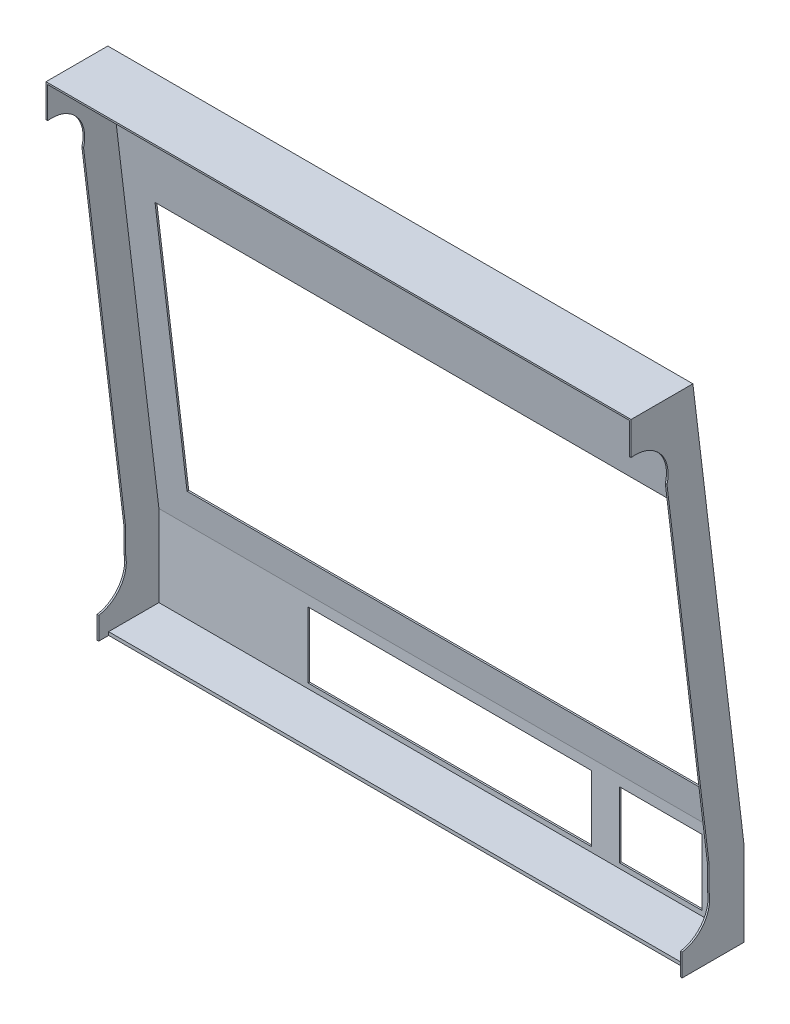
SolidWorks part; units mm, degrees
ref_plane "Front plane" through (0, 0, 0) normal (0, 0, 1) x (1, 0, 0)
ref_plane "Top plane" through (0, 0, 0) normal (0, 1, 0) x (1, 0, 0)
ref_plane "Right plane" through (0, 0, 0) normal (1, 0, 0) x (0, 0, -1)
sketch "Sketch1" plane through (0, 0, 0) normal (1, 0, 0) x (0, 0, -1)
  line L0 (0, 0) -> (-75, 0)
  line L1 (-75, 0) -> (-75, -40)
  line L2 (-13, -618) -> (-13, -590.821)
  line L3 (-31.4477, -90.1711) -> (19.6967, -515)
  line L4 (19.6967, -515) -> (19.6967, -543.6918)
  line L7 (-13, -618) -> (62, -618)
  line L8 (62, -618) -> (62, -515)
  line L9 (62, -515) -> (0, 0)
  arc A0 (-31.4477, -90.1711) -> (-75, -40) centre (-70.0509, -79.6926) ccw
  arc A1 (-13, -590.821) -> (19.6967, -543.6918) centre (-19.5608, -551.3627) ccw
  point P13 (62, -566.5)
  dimension "D3" = 42
  dimension "D7" = 80
  dimension "D8" = 80
  dimension "D1" = 75
  dimension "D2" = 40
  dimension "D4" = 618
  dimension "D5" = 103
  dimension "D6" = 137
extrude "Boss-Extrude1" add sketch "Sketch1" along normal blind 2
sketch "Sketch2" plane through (0, 0, 0) normal (-1, 0, 0) x (0, 0, 1)
  line L0 (-62, -618) -> (-62, -515) construction
  line L1 (-62, -515) -> (0, 0) construction
  line L2 (13, -618) -> (-62, -618) construction
  line L3 (0, 0) -> (75, 0) construction
  line L4 (13, -618) -> (-62, -618)
  line L5 (-62, -618) -> (-62, -515)
  line L6 (-62, -515) -> (0, 0)
  line L7 (0, 0) -> (75, 0)
  line L8 (13, -616) -> (-60, -616)
  line L9 (-60, -616) -> (-60, -515.12)
  line L10 (-60, -515.12) -> (1.7737, -2)
  line L11 (1.7737, -2) -> (75, -2)
  line L12 (13, -616) -> (13, -618)
  line L13 (75, 0) -> (75, -2)
  line L14 (75, -2) -> (75.2989, -2.0013)
  dimension "D1" = 2
extrude "Boss-Extrude2" add sketch "Sketch2" along normal blind 706 contours L11 L10 L9 L8 L12 L4 L5 L6 L7 L13
sketch "Sketch3" plane through (0, -616, 0) normal (0, 1, 0) x (1, 0, 0)
  line L4 (0, -13) -> (0, 60)
  line L5 (0, 60) -> (-706, 60)
  line L6 (-706, 60) -> (-706, -13)
  line L7 (-706, -13) -> (0, -13)
  line L8 (0, -13) -> (0, 60)
  line L9 (0, 60) -> (-706, 60)
  line L10 (-706, 60) -> (-706, -13)
  line L11 (-706, -13) -> (0, -13)
  dimension "D1" = 0
extrude "Cut-Extrude1" cut sketch "Sketch3" against normal through all
sketch "Sketch4" plane through (-706, 0, 0) normal (-1, 0, 0) x (0, 0, 1)
  line L8 (-19.6967, -543.6918) -> (-19.6967, -515)
  line L9 (-19.6967, -515) -> (31.4477, -90.1711)
  line L10 (75, -40) -> (75, 0)
  line L11 (75, 0) -> (0, 0)
  line L12 (0, 0) -> (-62, -515)
  line L13 (-62, -515) -> (-62, -618)
  line L14 (-62, -618) -> (13, -618)
  line L15 (13, -618) -> (13, -590.821)
  line L16 (-19.6967, -543.6918) -> (-19.6967, -515)
  line L17 (-19.6967, -515) -> (31.4477, -90.1711)
  line L18 (75, -40) -> (75, 0)
  line L19 (75, 0) -> (0, 0)
  line L20 (0, 0) -> (-62, -515)
  line L21 (-62, -515) -> (-62, -618)
  line L22 (-62, -618) -> (13, -618)
  line L23 (13, -618) -> (13, -590.821)
  arc A2 (-19.6967, -543.6918) -> (13, -590.821) centre (19.5608, -551.3627) ccw
  arc A3 (75, -40) -> (31.4477, -90.1711) centre (70.0509, -79.6926) ccw
  arc A4 (-19.6967, -543.6918) -> (13, -590.821) centre (19.5608, -551.3627) ccw
  arc A5 (75, -40) -> (31.4477, -90.1711) centre (70.0509, -79.6926) ccw
  dimension "D1" = 0
extrude "Boss-Extrude3" add sketch "Sketch4" along normal blind 2
sketch "Sketch5" plane through (0, 0, -62) normal (0, 0, -1) x (-1, 0, 0)
  line L0 (353, -618) -> (353, -180.8715) construction
  line L1 (-2, -618) -> (708, -618) construction
  line L2 (-2, -515) -> (708, -515) construction
  line L3 (39, -152) -> (667, -152)
  line L4 (39, -152) -> (39, -475)
  line L5 (39, -475) -> (667, -475)
  line L6 (667, -152) -> (667, -475)
  line L7 (39, -152) -> (667, -475) construction
  line L8 (39, -475) -> (667, -152) construction
  point P4 (353, -313.5)
  dimension "D1" = 323
  dimension "D2" = 40
  dimension "D3" = 628
extrude "Cut-Extrude2" cut sketch "Sketch5" against normal up to next
sketch "Sketch6" plane through (0, 0, -62) normal (0, 0, -1) x (-1, 0, 0)
  line L8 (147, -528) -> (47, -528)
  line L9 (147, -608) -> (147, -528)
  line L10 (47, -608) -> (147, -608)
  line L11 (47, -528) -> (47, -608)
  line L16 (525, -528) -> (181, -528)
  line L17 (525, -608) -> (525, -528)
  line L18 (181, -608) -> (525, -608)
  line L19 (181, -528) -> (181, -608)
extrude "Cut-Extrude3" cut sketch "Sketch6" against normal blind 2
sketch "Sketch7" plane through (0, 0, -60) normal (0, 0, 1) x (1, 0, 0)
  line L0 (0, -618) -> (0, -515.12) construction
  line L1 (-706, -618) -> (0, -618)
  line L2 (-706, -618) -> (-706, -614)
  line L3 (-706, -614) -> (0, -614)
  line L4 (0, -618) -> (0, -614)
  dimension "D1" = 4
extrude "Boss-Extrude4" add sketch "Sketch7" along normal blind 61
